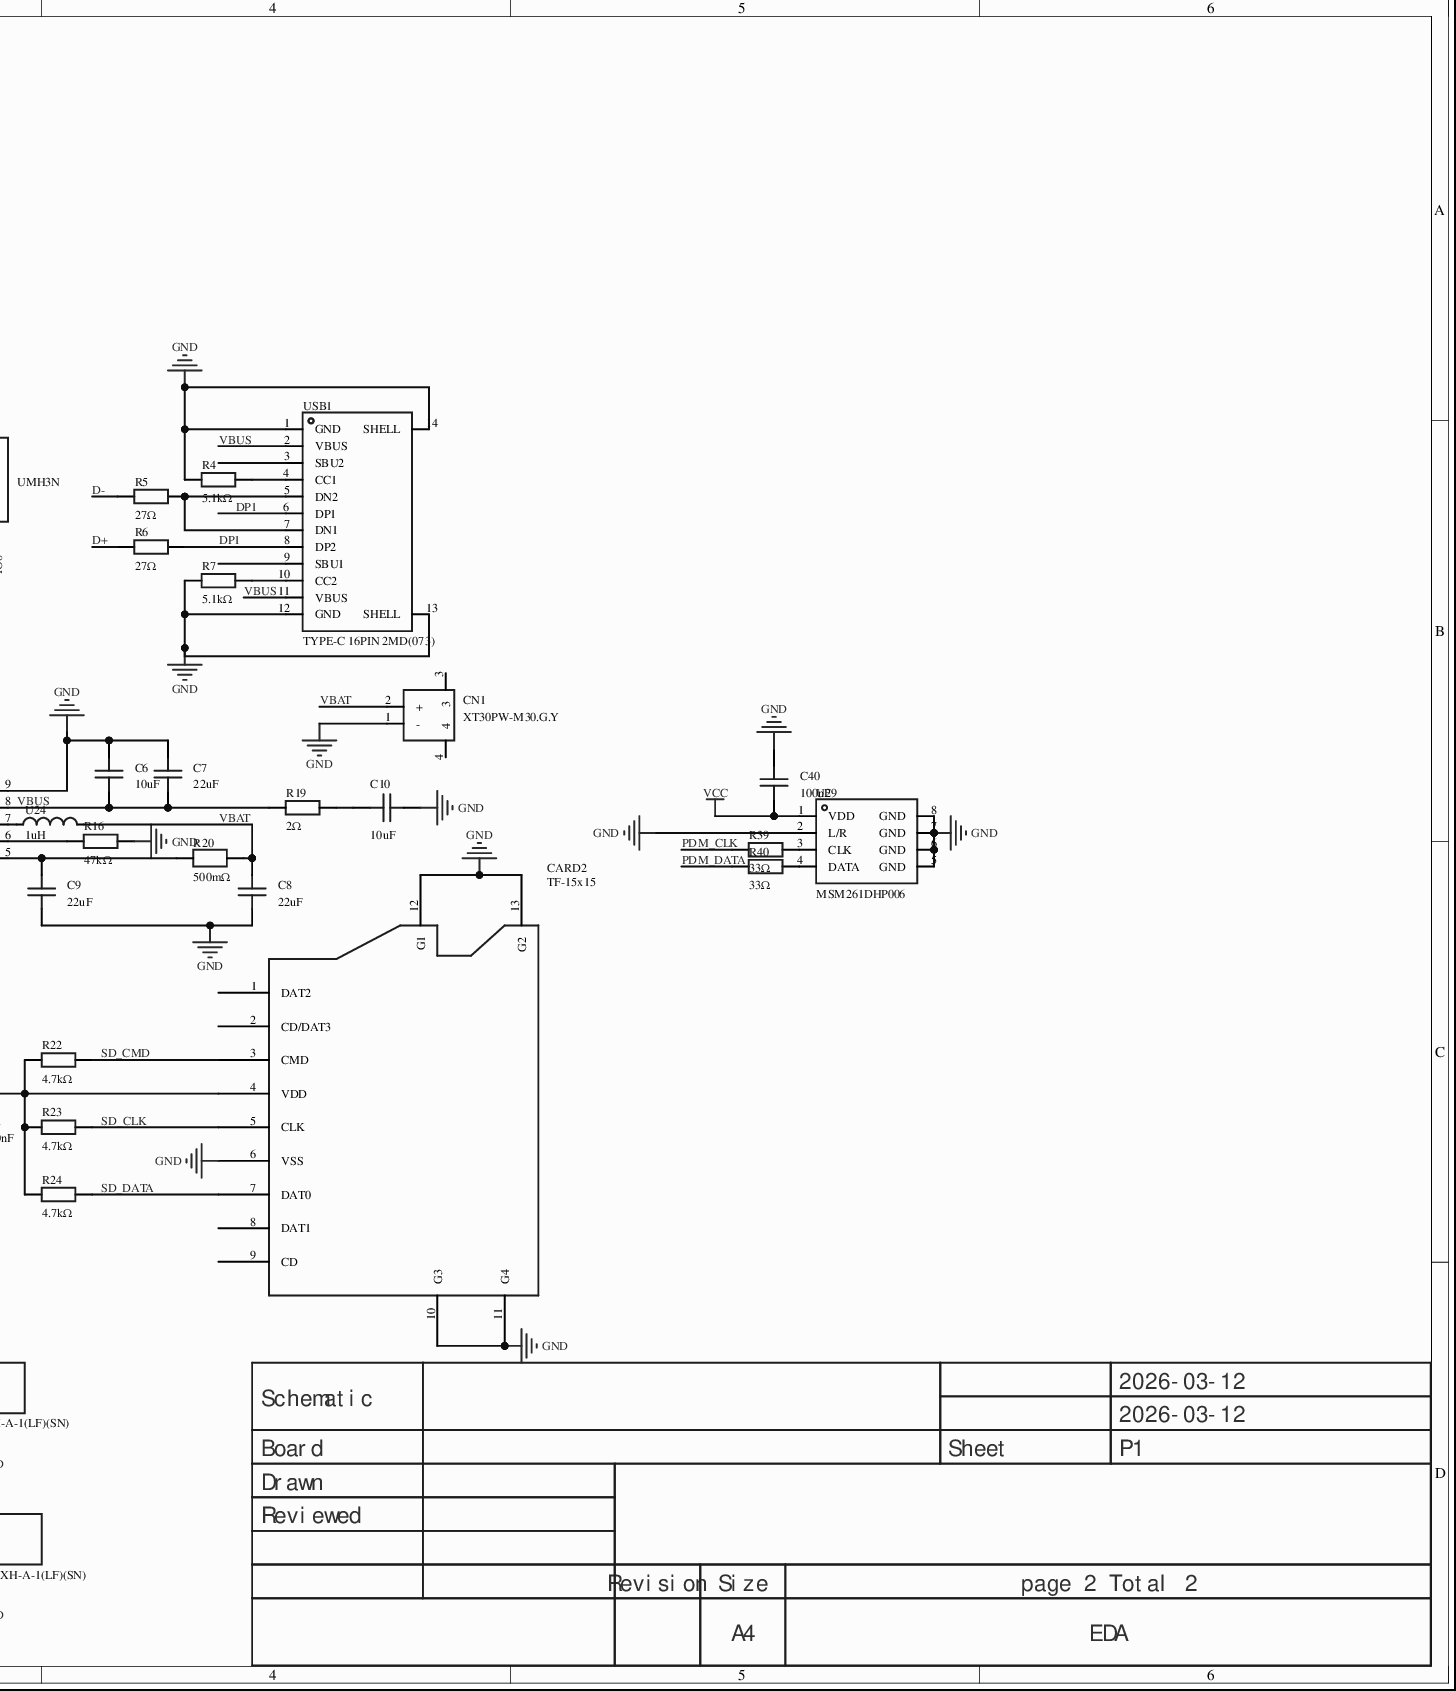
[diagram p0: MISC75432-3.schdoc, right]
# Altium project MISC75432-2.PrjPcb (part 2 of 3)

## Sheet MISC75432-3.schdoc (continued)

### Library data of the parts
C4 C5 = CL10C220JB8NNNC: Capacitance: 22pF; Tolerance: ±5%; Rated voltage: 50V; Temp. coefficient: C0G;; Manufacturer: SAMSUNG(三星); Add into BOM: yes; 3D Model: ac125912035d415993ca9572d50418b1; 3D Model Transform: 62.992,31.496,0,0,0,0,0,0,0; ModelName: C0603_L1.6-W0.8-H0.8; Symbol: CL10C220JB8NNNC; Device: CL10C220JB8NNNC; Convert to PCB: yes; Supplier Footprint: 0603; Value: 22pF; LCSC Part Name: 22pF ±5% 50V; Supplier Part: C1653; Manufacturer Part: CL10C220JB8NNNC; JLCPCB Part Class: Basic Part; Datasheet: https://example.com/datasheet/CL10C220JB8NNNC/2005.html; Supplier: LCSC; Voltage Rating: 50V; Temperature Coefficient: C0G; FootprintName: C0603
C6 C10 C15 C31 = CL10A106MA8NRNC: Capacitance: 10uF; Tolerance: ±20%; Rated voltage: 25V; Temp. coefficient: X5R;; Manufacturer: SAMSUNG(三星); Add into BOM: yes; 3D Model: ac125912035d415993ca9572d50418b1; 3D Model Transform: 62.992,31.496,0,0,0,0,0,0,0; ModelName: C0603_L1.6-W0.8-H0.8; Symbol: CL10A106MA8NRNC; Device: CL10A106MA8NRNC; Convert to PCB: yes; Supplier Footprint: 0603; Value: 10uF; LCSC Part Name: 10uF ±20% 25V; Supplier Part: C96446; Manufacturer Part: CL10A106MA8NRNC; JLCPCB Part Class: Basic Part; Datasheet: https://example.com/datasheet/CL10A106MA8NRNC/97651.html; Supplier: LCSC; Voltage Rating: 25V; Temperature Coefficient: X5R; FootprintName: C0603
C7-C9 C20 = CGA0603X5R226M160JT: Capacitance: 22uF; Tolerance: ±20%; Rated voltage: 16V; Temp. coefficient: X5R;; Manufacturer: HRE(芯声); Add into BOM: yes; 3D Model: ac125912035d415993ca9572d50418b1; 3D Model Transform: 62.992,31.496,0,0,0,0,0,0,0; ModelName: C0603_L1.6-W0.8-H0.8; Symbol: CGA0603X5R226M160JT; Device: CGA0603X5R226M160JT; Convert to PCB: yes; Supplier Footprint: 0603; Value: 22uF; LCSC Part Name: 22uF ±20% 16V; Supplier Part: C6119868; Manufacturer Part: CGA0603X5R226M160JT; JLCPCB Part Class: Extended Part; Datasheet: https://example.com/datasheet/CGA0603X5R226M160JT/7062574.html; Supplier: LCSC; Voltage Rating: 16V; Temperature Coefficient: X5R; FootprintName: C0603
C11 C12 C16 C18 C26 C32 C40 = CGA0603X7R104K500JT: Capacitance: 100nF; Tolerance: ±10%; Rated voltage: 50V; Temp. coefficient: X7R;; Manufacturer: HRE(芯声); Add into BOM: yes; 3D Model: ac125912035d415993ca9572d50418b1; 3D Model Transform: 62.992,31.496,0,0,0,0,0,0,0; ModelName: C0603_L1.6-W0.8-H0.8; Symbol: CGA0603X7R104K500JT; Device: CGA0603X7R104K500JT; Convert to PCB: yes; Supplier Footprint: 0603; Value: 100nF; LCSC Part Name: 100nF ±10% 50V; Supplier Part: C6119867; Manufacturer Part: CGA0603X7R104K500JT; JLCPCB Part Class: Extended Part; Datasheet: https://example.com/datasheet/CGA0603X7R104K500JT/7062573.html; Supplier: LCSC; Voltage Rating: 50V; Temperature Coefficient: X7R; FootprintName: C0603
C13 C14 C19 C27 C28 = CL10A105KB8NNNC: Capacitance: 1uF; Tolerance: ±10%; Rated voltage: 50V; Temp. coefficient: X5R;; Manufacturer: SAMSUNG(三星); Add into BOM: yes; 3D Model: ac125912035d415993ca9572d50418b1; 3D Model Transform: 62.992,31.496,0,0,0,0,0,0,0; ModelName: C0603_L1.6-W0.8-H0.8; Symbol: CL10A105KB8NNNC; Device: CL10A105KB8NNNC; Convert to PCB: yes; Supplier Footprint: 0603; Value: 1uF; LCSC Part Name: 1uF ±10% 50V; Supplier Part: C15849; Manufacturer Part: CL10A105KB8NNNC; JLCPCB Part Class: Basic Part; Datasheet: https://example.com/datasheet/CL10A105KB8NNNC/16531.html; Supplier: LCSC; Voltage Rating: 50V; Temperature Coefficient: X5R; FootprintName: C0603
C17 = RYHV50V2.2UF5*5: Capacitance: 2.2uF; Tolerance: ±20%; Rated voltage: 50V; Type: Polymer;; Manufacturer: HONOR(荣誉); Add into BOM: yes; 3D Model: ed942b427de741e3aabba01c64b2d723; 3D Model Transform: 236.22,208.661,0,0,0,0,-0.001,-0.003,0; Lifetime: 2000hrs@105℃; Symbol: RYHV50V2.2UF5*5; Device: RYHV50V2.2UF5*5; Convert to PCB: yes; Supplier Footprint: SMD,D5xL5.8mm; Value: 2.2uF; LCSC Part Name: 2.2uF ±20% 50V; Supplier Part: C48970657; Manufacturer Part: RYHV50V2.2UF5*5; JLCPCB Part Class: Extended Part; Datasheet: https://example.com/datasheet/RYHV50V2.2UF5*5/51295601.html; Supplier: LCSC; Voltage Rating: 50V; Type: Polymer; Diameter: 5mm; Height - Seated (Max): 5.8mm; Operating Temperature: -55℃~+105℃; FootprintName: CAP-SMD_BD5.0-L5.3-W5.3-LS6.0-FD; ModelName: CAP-SMD_BD5.0-L5.3-W5.3-LS6.0-FD
C21 = CL10C330JB8NNNC: Capacitance: 33pF; Tolerance: ±5%; Rated voltage: 50V; Temp. coefficient: C0G;; Manufacturer: SAMSUNG(三星); Add into BOM: yes; 3D Model: ac125912035d415993ca9572d50418b1; 3D Model Transform: 62.992,31.496,0,0,0,0,0,0,0; ModelName: C0603_L1.6-W0.8-H0.8; Symbol: CL10C330JB8NNNC; Device: CL10C330JB8NNNC; Convert to PCB: yes; Supplier Footprint: 0603; Value: 33pF; LCSC Part Name: 33pF ±5% 50V; Supplier Part: C1663; Manufacturer Part: CL10C330JB8NNNC; JLCPCB Part Class: Basic Part; Datasheet: https://example.com/datasheet/CL10C330JB8NNNC/2015.html; Supplier: LCSC; Voltage Rating: 50V; Temperature Coefficient: C0G; FootprintName: C0603
C22 = CL10B473KB8NNNC: Capacitance: 47nF; Tolerance: ±10%; Rated voltage: 50V; Temp. coefficient: X7R;; Manufacturer: SAMSUNG(三星); Add into BOM: yes; 3D Model: ac125912035d415993ca9572d50418b1; 3D Model Transform: 62.992,31.496,0,0,0,0,0,0,0; ModelName: C0603_L1.6-W0.8-H0.8; Symbol: CL10B473KB8NNNC; Device: CL10B473KB8NNNC; Convert to PCB: yes; Supplier Footprint: 0603; Value: 47nF; LCSC Part Name: 47nF ±10% 50V; Supplier Part: C1622; Manufacturer Part: CL10B473KB8NNNC; JLCPCB Part Class: Basic Part; Datasheet: https://example.com/datasheet/CL10B473KB8NNNC/1974.html; Supplier: LCSC; Voltage Rating: 50V; Temperature Coefficient: X7R; FootprintName: C0603
C23-C25 = RVT25V22M5X5: Capacitance: 22uF; Tolerance: ±20%; Rated voltage: 25V; Ripple current: 26mA@120Hz;; Manufacturer: JIERR(捷而瑞); AddInBom: yes; ModelId: 95a10e3217cd46fe9ce33b4e001305500819f05c4eef4c71ace90d822a990e87; ModelTransform: 224.409,208.661,0,0,0,0,0,0,0; Lifetime: 2000hrs@105℃; Symbol: RVT25V22M5X5; Device: RVT25V22M5X5; LCSC Part Name: 22uF ±20% 25V; SupplierPart: C47023110; ManufacturerPart: RVT25V22M5X5; Supplier Footprint: SMD,D5xL5.4mm; JLCPCB Part Class: Extended Part; Datasheet: https://example.com/datasheet/RVT25V22M5X5/49206211.html; Supplier: LCSC; ConvertToPcb: yes; FootprintName: CAP-SMD_BD5.0-L5.3-W5.3-LS6.3-FD-1; ModelName: CAP-SMD_BD5.0-L5.3-W5.3-LS6.3-FD-1; Value: 22uF; Voltage Rating: 25V; Ripple Current: 26mA@120Hz; Diameter: 5mm; Height - Seated (Max): 5.4mm; Operating Temperature: -55℃~+105℃
C29 = JVJ25V220M6x8: Capacitance: 220uF; Tolerance: ±20%; Rated voltage: 25V; Ripple current: 120mA@120Hz;; Manufacturer: JIERR(捷而瑞); AddInBom: yes; ModelId: ccbda52dceed4b139172c40f75c9da3f0819f05c4eef4c71ace90d822a990e87; ModelTransform: 287.401,259.842,0,0,0,0,0,0,0; Lifetime: 2000hrs@105℃; Symbol: JVJ25V220M6X8; Device: JVJ25V220M6x8; LCSC Part Name: 220uF ±20% 25V; SupplierPart: C46550404; ManufacturerPart: JVJ25V220M6x8; Supplier Footprint: SMD,D6.3xL7.7mm; JLCPCB Part Class: Extended Part; Datasheet: https://example.com/datasheet/JVJ25V220M6x8/48680098.html; Supplier: LCSC; ConvertToPcb: yes; FootprintName: CAP-SMD_BD6.3-L6.6-W6.6-LS7.3-FD-H7.7; ModelName: CAP-SMD_BD6.3-L6.6-W6.6-LS7.3-FD-H7.7; Value: 220uF; Voltage Rating: 25V; Ripple Current: 120mA@120Hz; Diameter: 6.3mm; Height - Seated (Max): 7.7mm; Operating Temperature: -55℃~+105℃
C30 C37-C39 = CC0603KRX7R7BB684: Capacitance: 680nF; Tolerance: ±10%; Rated voltage: 16V; Temp. coefficient: X7R;; Manufacturer: YAGEO(国巨); Add into BOM: yes; 3D Model: ac125912035d415993ca9572d50418b1; 3D Model Transform: 62.992,31.496,0,0,0,0,0,0,0; ModelName: C0603_L1.6-W0.8-H0.8; Symbol: CC0603KRX7R7BB684; Device: CC0603KRX7R7BB684; Convert to PCB: yes; Supplier Footprint: 0603; Value: 680nF; LCSC Part Name: 680nF ±10% 16V; Supplier Part: C107067; Manufacturer Part: CC0603KRX7R7BB684; JLCPCB Part Class: Extended Part; Datasheet: https://example.com/datasheet/CC0603KRX7R7BB684/108283.html; Supplier: LCSC; Voltage Rating: 16V; Temperature Coefficient: X7R; FootprintName: C0603
C33-C36 = CL10B224KA8NNNC: Capacitance: 220nF; Tolerance: ±10%; Rated voltage: 25V; Temp. coefficient: X7R;; Manufacturer: SAMSUNG(三星); Add into BOM: yes; 3D Model: ac125912035d415993ca9572d50418b1; 3D Model Transform: 62.992,31.496,0,0,0,0,0,0,0; ModelName: C0603_L1.6-W0.8-H0.8; Symbol: CL10B224KA8NNNC; Device: CL10B224KA8NNNC; Convert to PCB: yes; Supplier Footprint: 0603; Value: 220nF; LCSC Part Name: 220nF ±10% 25V; Supplier Part: C21120; Manufacturer Part: CL10B224KA8NNNC; JLCPCB Part Class: Basic Part; Datasheet: https://example.com/datasheet/CL10B224KA8NNNC/21832.html; Supplier: LCSC; Voltage Rating: 25V; Temperature Coefficient: X7R; FootprintName: C0603
C41 = CL10B102KB8NNNC: Capacitance: 1nF; Tolerance: ±10%; Rated voltage: 50V; Temp. coefficient: X7R;; Manufacturer: SAMSUNG(三星); Add into BOM: yes; 3D Model: ac125912035d415993ca9572d50418b1; 3D Model Transform: 62.992,31.496,0,0,0,0,0,0,0; ModelName: C0603_L1.6-W0.8-H0.8; Symbol: CL10B102KB8NNNC; Device: CL10B102KB8NNNC; Convert to PCB: yes; Supplier Footprint: 0603; Value: 1nF; LCSC Part Name: 1nF ±10% 50V; Supplier Part: C1588; Manufacturer Part: CL10B102KB8NNNC; JLCPCB Part Class: Basic Part; Datasheet: https://example.com/datasheet/CL10B102KB8NNNC/1940.html; Supplier: LCSC; Voltage Rating: 50V; Temperature Coefficient: X7R; FootprintName: C0603
CARD2 = TF-15x15: Card connection: Self-ejecting; Card type: MicroSD card (TF card); Connector type: Socket; Max body height: 2mm; Operating temp.: -25℃~+85℃;; Manufacturer: SOFNG(硕方); Symbol: TF-15×15; AddInBom: yes; ModelId: 67496f576e2f431c95a797a452f0eadc0819f05c4eef4c71ace90d822a990e87; ModelTransform: 598.424,635.826,0,0,0,0,79.804,8.934,-23.622; Device: TF-15x15; LCSC Part Name: 自弹式 MicroSD卡(TF卡) 卡座; SupplierPart: C111196; ManufacturerPart: TF-15x15; Supplier Footprint: SMD; JLCPCB Part Class: Extended Part; Datasheet: https://example.com/datasheet/TF-15x15/112422.html; Supplier: LCSC; ConvertToPcb: yes; FootprintName: TF-SMD_TF-15-15; ModelName: TF-SMD_TF-15-15; Card Connection Mode: Self-ejecting; Card Type: MicroSD card (TF card); Connector Type: Socket; Additional Card Detection Pins: Yes; Height Above Board: 2mm; Operating Temperature: -25℃~+85℃
CN1 = XT30PW-M30.G.Y: Socket,DCsupply,XT30,male,PIN:2; Manufacturer: AMASS(艾迈斯); AddInBom: yes; ModelId: 722652c2597f41cd937322584dc4b29b0819f05c4eef4c71ace90d822a990e87; ModelTransform: 523.621,549.2115,0,0,0,0,-0.005,-39.568,-78.74; Rated current: 15A; Rated voltage: 500VDC; Connector type: RC model plug; Wire gauge: 16/18/20AWG; contact resistance: 1.2mΩ; Symbol: XT30PW-M; Device: XT30PW-M30.G.Y; LCSC Part Name: AMASS(艾迈斯)航模插头 卧式弯脚 XT30PW-M公头; SupplierPart: C431092; ManufacturerPart: XT30PW-M30.G.Y; Supplier Footprint: -; JLCPCB Part Class: Extended Part; Datasheet: https://example.com/datasheet/XT30PW-M30.G.Y/426930.html; Supplier: LCSC; ConvertToPcb: yes; FootprintName: CONN-TH_XT30PW-M; ModelName: CONN-TH_XT30PW-M; Size/Specification: 2pin; interface form: Male
CN2 CN3 = S2B-XH-A-1(LF)(SN): Pin structure: 1x2P; Pitch: 2.5mm; Mounting: Right-angle THT; Series: XH; Total pins: 2P; Rows: 1; Pins per row: 2; Row spacing: -; Rated current: 3A; Contact material: Brass; Contact plating: Tin; Operating temp.: -25℃~+85℃;; Manufacturer: JST; AddInBom: yes; ModelId: 91927f2a0f7340abaa498c02c76d9b390819f05c4eef4c71ace90d822a990e87; ModelTransform: 291.338,452.755,0,0,0,0,0.394,73.43,-129.921; Number of PINs Per Row: 2; Voltage Rating: 250V; Plastic Material: PA66; Flame Retardant Rating: UL94V-0; Supplementary Features: Kinked pins; Z-Height of the Board: 6.1mm; X-Length of Bottom Edge on Board (Spacing Line): 7.4mm; Y-Width of Bottom Edge on Board: 11.5mm; Symbol: S2B-XH-A-1 (LF)(SN); Device: S2B-XH-A-1(LF)(SN); LCSC Part Name: 1x2P 间距:2.5mm 弯插 系列:XH; SupplierPart: C163035; ManufacturerPart: S2B-XH-A-1(LF)(SN); Supplier Footprint: 弯插,P=2.5mm; JLCPCB Part Class: Extended Part; Datasheet: https://example.com/datasheet/S2B-XH-A-1(LF)(SN)/174416.html; Supplier: LCSC; ConvertToPcb: yes; FootprintName: CONN-TH_S2B-XH-A-1-LF-SN; ModelName: CONN-TH_S2B-XH-A-1-LF-SN; Pins Structure: 1x2P; Mounting Type: Right-angle THT; Reference Series: XH; Number of Pins: 2P; Number of Rows: 1; Row Spacing: -; Current Rating: 3A; Contact Material: Brass; Contact Plating: Tin; Operating Temperature: -25℃~+85℃; Color: White
D1 D2 = 1N4148W_C7420318: Diode configuration: Discrete; Forward voltage drop (Vf): 1.25V@150mA; DC reverse voltage (Vr): 100V; Rectified current: 150mA; Reverse recovery time (Trr): 4ns;; Manufacturer: R+O(宏嘉诚); AddInBom: yes; ModelId: 5054d9b7be8b429dad093a54b517b4dd0819f05c4eef4c71ace90d822a990e87; ModelTransform: 145.669,61.024,0,0,0,0,0,0,0; Pd - Power Dissipation: 400mW; Reverse Leakage Current (Ir): 1uA@75V; Operating Junction Temperature Range: -55℃~+150℃; Non-Repetitive Peak Forward Surge Current: 2A; Symbol: 1N4148W_C7420318; Device: 1N4148W_C7420318; LCSC Part Name: 100V 150mA; SupplierPart: C7420318; ManufacturerPart: 1N4148W; Supplier Footprint: SOD-123; JLCPCB Part Class: Extended Part; Datasheet: https://example.com/datasheet/1N4148W/8397140.html; Supplier: LCSC; ConvertToPcb: yes; FootprintName: SOD-123_L2.7-W1.6-LS3.7-FD; ModelName: SOD-123_L2.7-W1.6-LS3.7-FD; Diode Configuration: Discrete; Voltage - Forward(Vf@If): 1.25V@150mA; Voltage - DC Reverse(Vr): 100V; Current - Rectified: 150mA; Reverse Recovery Time (trr): 4ns
L1 = SRG0420-2R2-M: Inductance: 2.2uH; Tolerance: ±20%; Rated current: 4A; Saturation current (Isat): 5A; Type: Molded inductor;; Manufacturer: JIERR(捷而瑞); AddInBom: yes; DC Resistance(DCR): 49mΩ; Symbol: SRG0420-2R2-M; Device: SRG0420-2R2-M; LCSC Part Name: 2.2μH ±20% 5A; SupplierPart: C53462916; ManufacturerPart: SRG0420-2R2-M; Supplier Footprint: SMD,4.6x4.1mm; JLCPCB Part Class: Extended Part; Datasheet: https://example.com/datasheet/SRG0420-2R2-M/56628161.html; Supplier: LCSC; ConvertToPcb: yes; FootprintName: IND-SMD_L4.6-W4.1_MHCI04015; Value: 2.2uH; Current Rating: 4A; Current - Saturation(Isat): 5A; Type: Molded inductor
L2-L5 = FXL0630-100-M: Inductance: 10uH; Tolerance: ±20%; Rated current: 4.5A; Saturation current (Isat): 5.5A; Type: Molded inductor;; Manufacturer: cjiang(长江微电); AddInBom: yes; ModelId: e28854526ca747668ea12fbe1dd39a630819f05c4eef4c71ace90d822a990e87; ModelName: IND-SMD_L7.3-W6.8-H3.0; ModelTransform: 292.125,267.716,0,0,0,0,0,0,0; DC Resistance(DCR): 68mΩ; Symbol: FXL0630-100-M; Device: FXL0630-100-M; LCSC Part Name: 10uH ±20% 5.5A; SupplierPart: C167223; ManufacturerPart: FXL0630-100-M; Supplier Footprint: SMD,7x6.6mm; JLCPCB Part Class: Extended Part; Datasheet: https://example.com/datasheet/FXL0630-100-M/178606.html; Supplier: LCSC; ConvertToPcb: yes; FootprintName: IND-SMD_L7.3-W6.8; Value: 10uH; Current Rating: 4.5A; Current - Saturation(Isat): 5.5A; Type: Molded inductor; Ratings: -
LED1 LED2 = NCD0603Y2: Emitted color: Yellow; Forward voltage (VF): 1.6V~2.6V; Power: 65mW; Forward current: 20mA; Dominant wavelength: 586nm~595nm; Lens color: Clear lens; Luminous intensity: 100mcd~220mcd; Viewing angle: 130°; Operating temp.: -30℃~+85℃;; Manufacturer: 国星光电; Symbol: FC-1608YXK-585F08; AddInBom: yes; ModelId: 1f0d29a91be547639d425604e9b96ebb0819f05c4eef4c71ace90d822a990e87; ModelTransform: 63.7794,32.283,0,0,0,0,0,0,0; Device: NCD0603Y2; LCSC Part Name: NCD0603Y2; SupplierPart: C89811; ManufacturerPart: NCD0603Y2; Supplier Footprint: 0603; JLCPCB Part Class: Extended Part; Datasheet: https://example.com/upload/public/pdf/source/20200820/C89811_7FE84B429B6BCA3E113B125EE1452576.pdf; Supplier: LCSC; ConvertToPcb: yes; FootprintName: LED0603-RD; ModelName: LED0603-RD; Emitted Color: Yellow; Forward Voltage (VF): 1.6V~2.6V; Power Dissipation: 65mW; Forward Current: 20mA; Dominant Wavelength: 586nm~595nm; Lens Color: Clear lens; Luminous Intensity: 100mcd~220mcd; Viewing Angle: 130°; Operating Temperature: -30℃~+85℃
Q17 = UMH3N: Quantity: -; Collector-emitter breakdown voltage (Vceo): 50V; Collector current (Ic): 100mA; Power dissipation (Pd): 150mW; DC current gain (hFE): 100@1mA,5V;; Manufacturer: CJ(江苏长电/长晶); AddInBom: yes; ModelId: 7779600a2eb94c6fae04993c10cd58cb0819f05c4eef4c71ace90d822a990e87; ModelName: SC-70-6_L2.0-W1.3-H1.0-P0.65; ModelTransform: 82.677,78.74,0,0,0,0,0,0,0; Input Resistor: 6.11kΩ; Symbol: UMH3N; Device: UMH3N; LCSC Part Name: 数字晶体管（内置电阻）; SupplierPart: C62892; ManufacturerPart: UMH3N; Supplier Footprint: SOT-363; JLCPCB Part Class: Extended Part; Datasheet: https://example.com/datasheet/UMH3N/63955.html; Supplier: LCSC; ConvertToPcb: yes; FootprintName: SC-70-6_L2.2-W1.3-P0.65-LS2.1-BR; Number: -; Collector - Emitter Voltage VCEO: 50V; Current - Collector(Ic): 100mA; Pd - Power Dissipation: 150mW; DC Current Gain: 100@1mA,5V; Emitter-Base Voltage VEBO: 5V; Operating Temperature: -55℃~+150℃
Q18 = 2N7002_C8545: Quantity: 1 N-channel; Drain-source voltage (Vdss): 60V; Continuous drain current (Id): 115mA; On-resistance (RDS(on)): 5Ω@10V; Power dissipation (Pd): 225mW; Threshold voltage (Vgs(th)): 2.5V;; Manufacturer: CJ(江苏长电/长晶); 3D Model: c62791f0466c4ae2a892c056b845b0ca0819f05c4eef4c71ace90d822a990e87; 3D Model Transform: 98.425,114.173,0,180,0,0,0.0005,-0.0005,0; Input Capacitance(Ciss): 50pF; Reverse Transfer Capacitance (Crss@Vds): 5pF; AddInBom: yes; ModelName: SOT-23-3P_L2.9-W1.3-H1.0-LS2.4-P0.95; Symbol: 2N7002; Device: 2N7002_C8545; LCSC Part Name: 1个N沟道 耐压:60V 电流:115mA; Supplier Part: C8545; Manufacturer Part: 2N7002; Supplier Footprint: SOT-23; JLCPCB Part Class: Basic Part; Datasheet: https://example.com/datasheet/2N7002/9040.html; Supplier: LCSC; Number: 1 N-channel; Drain to Source Voltage: 60V; Current - Continuous Drain(Id): 115mA; RDS(on): 5Ω@10V; Pd - Power Dissipation: 225mW; Gate Threshold Voltage (Vgs(th)): 2.5V; Operating Temperature: -; ConvertToPcb: yes; FootprintName: SOT-23-3_L2.9-W1.3-P1.90-LS2.4-BR
R3 R13 R26 R34 R36 = 0603WAF1002T5E: Resistor type: Thick-film; Resistance: 10kΩ; Tolerance: ±1%; Power: 100mW; Working voltage: 75V; Temp. coefficient: ±100ppm/℃;; Manufacturer: UNI-ROYAL(厚声); Add into BOM: yes; 3D Model: fc143cca1e79419f9cd78b61e9279f08; 3D Model Transform: 31.8897,63.7794,0,90,0,0,0,0,0; Symbol: 0603WAF1002T5E; Device: 0603WAF1002T5E; Convert to PCB: yes; Supplier Footprint: 0603; Value: 10kΩ; LCSC Part Name: 厚膜电阻 10kΩ ±1% 100mW; Supplier Part: C25804; Manufacturer Part: 0603WAF1002T5E; JLCPCB Part Class: Basic Part; Datasheet: https://example.com/datasheet/0603WAF1002T5E/26547.html; Supplier: LCSC; Type: Thick-film resistor; Power(Watts): 100mW; Voltage-Supply(Max): 75V; Temperature Coefficient: ±100ppm/℃; Operating Temperature: -55℃~+155℃; FootprintName: R0603; ModelName: R0603
R4 R7 = 0603WAF5101T5E: Resistor type: Thick-film; Resistance: 5.1kΩ; Tolerance: ±1%; Power: 100mW; Working voltage: 75V; Temp. coefficient: ±100ppm/℃;; Manufacturer: UNI-ROYAL(厚声); Add into BOM: yes; 3D Model: fc143cca1e79419f9cd78b61e9279f08; 3D Model Transform: 31.8897,63.7794,0,90,0,0,0,0,0; Symbol: 0603WAF5101T5E; Device: 0603WAF5101T5E; Convert to PCB: yes; Supplier Footprint: 0603; Value: 5.1kΩ; LCSC Part Name: 5.1kΩ ±1% 100mW 厚膜电阻; Supplier Part: C23186; Manufacturer Part: 0603WAF5101T5E; JLCPCB Part Class: Basic Part; Datasheet: https://example.com/datasheet/0603WAF5101T5E/23913.html; Supplier: LCSC; Type: Thick-film resistor; Power(Watts): 100mW; Voltage-Supply(Max): 75V; Temperature Coefficient: ±100ppm/℃; Operating Temperature: -55℃~+155℃; FootprintName: R0603; ModelName: R0603
R5 R6 = 0603WAF270JT5E: Resistor type: Thick-film; Resistance: 27Ω; Tolerance: ±1%; Power: 100mW; Working voltage: 75V; Temp. coefficient: ±200ppm/℃;; Manufacturer: UNI-ROYAL(厚声); Add into BOM: yes; 3D Model: fc143cca1e79419f9cd78b61e9279f08; 3D Model Transform: 31.8897,63.7794,0,90,0,0,0,0,0; Symbol: 0603WAF270JT5E; Device: 0603WAF270JT5E; Convert to PCB: yes; Supplier Footprint: 0603; Value: 27Ω; LCSC Part Name: 27Ω ±1% 100mW 厚膜电阻; Supplier Part: C25190; Manufacturer Part: 0603WAF270JT5E; JLCPCB Part Class: Extended Part; Datasheet: https://example.com/datasheet/0603WAF270JT5E/25933.html; Supplier: LCSC; Type: Thick-film resistor; Power(Watts): 100mW; Voltage-Supply(Max): 75V; Temperature Coefficient: ±200ppm/℃; Operating Temperature: -55℃~+155℃; FootprintName: R0603; ModelName: R0603
R8-R12 = FRC0603F49R9TS: Resistor type: Thick-film; Resistance: 49.9Ω; Tolerance: ±1%; Power: 100mW; Working voltage: 75V; Temp. coefficient: ±100ppm/℃;; Manufacturer: FOJAN(富捷); Add into BOM: yes; 3D Model: fc143cca1e79419f9cd78b61e9279f08; 3D Model Transform: 31.8897,63.7794,0,90,0,0,0,0,0; Symbol: FRC0603F49R9TS; Device: FRC0603F49R9TS; Convert to PCB: yes; Supplier Footprint: 0603; Value: 49.9Ω; LCSC Part Name: 49.9Ω ±1% 100mW 厚膜电阻; Supplier Part: C2930110; Manufacturer Part: FRC0603F49R9TS; JLCPCB Part Class: Extended Part; Supplier: LCSC; Type: Thick-film resistor; Power(Watts): 100mW; Voltage-Supply(Max): 75V; Temperature Coefficient: ±100ppm/℃; Operating Temperature: -55℃~+155℃; FootprintName: R0603; ModelName: R0603
R14 = 0603WAF1001T5E: Resistor type: Thick-film; Resistance: 1kΩ; Tolerance: ±1%; Power: 100mW; Working voltage: 75V; Temp. coefficient: ±100ppm/℃;; Manufacturer: UNI-ROYAL(厚声); Add into BOM: yes; 3D Model: fc143cca1e79419f9cd78b61e9279f08; 3D Model Transform: 31.8897,63.7794,0,90,0,0,0,0,0; Symbol: 0603WAF1001T5E; Device: 0603WAF1001T5E; Convert to PCB: yes; Supplier Footprint: 0603; Value: 1kΩ; LCSC Part Name: 1kΩ ±1% 100mW 厚膜电阻; Supplier Part: C21190; Manufacturer Part: 0603WAF1001T5E; JLCPCB Part Class: Basic Part; Datasheet: https://example.com/datasheet/0603WAF1001T5E/21904.html; Supplier: LCSC; Type: Thick-film resistor; Power(Watts): 100mW; Voltage-Supply(Max): 75V; Temperature Coefficient: ±100ppm/℃; Operating Temperature: -55℃~+155℃; FootprintName: R0603; ModelName: R0603
R15 = 0603WAF8202T5E: Resistor type: Thick-film; Resistance: 82kΩ; Tolerance: ±1%; Power: 100mW; Working voltage: 75V; Temp. coefficient: ±100ppm/℃;; Manufacturer: UNI-ROYAL(厚声); Add into BOM: yes; 3D Model: fc143cca1e79419f9cd78b61e9279f08; 3D Model Transform: 31.8897,63.7794,0,90,0,0,0,0,0; Symbol: 0603WAF8202T5E; Device: 0603WAF8202T5E; Convert to PCB: yes; Supplier Footprint: 0603; Value: 82kΩ; LCSC Part Name: 82kΩ ±1% 100mW 厚膜电阻; Supplier Part: C23254; Manufacturer Part: 0603WAF8202T5E; JLCPCB Part Class: Basic Part; Datasheet: https://example.com/datasheet/0603WAF8202T5E/23981.html; Supplier: LCSC; Type: Thick-film resistor; Power(Watts): 100mW; Voltage-Supply(Max): 75V; Temperature Coefficient: ±100ppm/℃; Operating Temperature: -55℃~+155℃; FootprintName: R0603; ModelName: R0603
R16 = 0603WAF4702T5E: Resistor type: Thick-film; Resistance: 47kΩ; Tolerance: ±1%; Power: 100mW; Working voltage: 75V; Temp. coefficient: ±100ppm/℃;; Manufacturer: UNI-ROYAL(厚声); Add into BOM: yes; 3D Model: fc143cca1e79419f9cd78b61e9279f08; 3D Model Transform: 31.8897,63.7794,0,90,0,0,0,0,0; Symbol: 0603WAF4702T5E; Device: 0603WAF4702T5E; Convert to PCB: yes; Supplier Footprint: 0603; Value: 47kΩ; LCSC Part Name: 47kΩ ±1% 100mW 厚膜电阻; Supplier Part: C25819; Manufacturer Part: 0603WAF4702T5E; JLCPCB Part Class: Basic Part; Datasheet: https://example.com/datasheet/0603WAF4702T5E/26562.html; Supplier: LCSC; Type: Thick-film resistor; Power(Watts): 100mW; Voltage-Supply(Max): 75V; Temperature Coefficient: ±100ppm/℃; Operating Temperature: -55℃~+155℃; FootprintName: R0603; ModelName: R0603
R17 R21 = 0603WAF1000T5E: Resistor type: Thick-film; Resistance: 100Ω; Tolerance: ±1%; Power: 100mW; Max working voltage: 75V; Temp. coefficient: ±200ppm/℃;; Manufacturer: UNI-ROYAL(厚声); Add into BOM: yes; 3D Model: fc143cca1e79419f9cd78b61e9279f08; 3D Model Transform: 31.8897,63.7794,0,90,0,0,0,0,0; Symbol: 0603WAF1000T5E; Device: 0603WAF1000T5E; Convert to PCB: yes; Supplier Footprint: 0603; Value: 100Ω; LCSC Part Name: 100Ω ±1% 100mW 厚膜电阻; Supplier Part: C22775; Manufacturer Part: 0603WAF1000T5E; JLCPCB Part Class: Basic Part; Datasheet: https://example.com/upload/public/pdf/source/20200306/C422600_1E6D84923E4A46A82E41ADD87F860B5C.pdf; Supplier: LCSC; Type: Thick-film resistor; Power(Watts): 100mW; Overload Voltage (Max): 75V; Temperature Coefficient: ±200ppm/℃; Operating Temperature Range: -55℃~+155℃; FootprintName: R0603; ModelName: R0603
R18 = HNTC0805-104F3950FB: Resistance: 100kΩ; B value (25℃/50℃): 3950K; Resistance tolerance: ±1%; Power: 200mW; B value tolerance: ±1%; Max steady-state current (25℃): 140uA;; Manufacturer: R+O(宏嘉诚); AddInBom: yes; ModelId: 37a81e68749a4138bd2dfa6897b24b850819f05c4eef4c71ace90d822a990e87; ModelName: R0805_L2.0-W1.3-H0.6; ModelTransform: 78.74,51.181,0,0,0,0,0,-0.0005,0; Dissipation Factor: 2mW/℃; Thermal Time Constant: 5s; Pitch: 0.5mm; Symbol: HNTC0805-104F3950FB; Device: HNTC0805-104F3950FB; LCSC Part Name: HNTC0805-104F3950FB; SupplierPart: C49247664; ManufacturerPart: HNTC0805-104F3950FB; Supplier Footprint: 0805; JLCPCB Part Class: Extended Part; Datasheet: https://example.com/datasheet/HNTC0805-104F3950FB/51678317.html; Supplier: LCSC; ConvertToPcb: yes; FootprintName: R0805; Resistance @ 25℃: 100kΩ; B Constant (25℃/50℃): 3950K; Resistance Tolerance: ±1%; Power(Watts): 200mW; B Constant Tolerance: ±1%; Steady State Current (Max): 140uA; Operating Temperature: -40℃~+125℃; Length: 2mm; Width: 1.25mm; Height: 0.85mm
R19 = RC0603FR-072RL: Resistor type: Thick-film; Resistance: 2Ω; Tolerance: ±1%; Power: 100mW; Max working voltage: 75V; Temp. coefficient: ±200ppm/℃;; Manufacturer: YAGEO(国巨); Add into BOM: yes; 3D Model: fc143cca1e79419f9cd78b61e9279f08; 3D Model Transform: 31.8897,63.7794,0,90,0,0,0,0,0; Symbol: RC0603FR-072RL; Device: RC0603FR-072RL; Convert to PCB: yes; Supplier Footprint: 0603; Value: 2Ω; LCSC Part Name: 厚膜电阻 2Ω ±1% 100mW; Supplier Part: C185341; Manufacturer Part: RC0603FR-072RL; JLCPCB Part Class: Extended Part; Datasheet: https://example.com/upload/public/pdf/source/20180904/C276339_014E484F1DBA106FB92D45EABD5A1AC1.pdf; Supplier: LCSC; Type: Thick-film resistor; Power(Watts): 100mW; Overload Voltage (Max): 75V; Temperature Coefficient: ±200ppm/℃; Operating Temperature Range: -55℃~+155℃; FootprintName: R0603; ModelName: R0603
R20 = HoJLRH1206-1W-500mR-1%: Resistor type: Thin-film; Resistance: 500mΩ; Tolerance: ±1%; Power: 1W; Temp. coefficient: ±100ppm/℃;; Manufacturer: Milliohm(毫欧); AddInBom: yes; ModelId: 89a1f13db2384da588040e0b3c55bf660819f05c4eef4c71ace90d822a990e87; ModelName: R1206_L3.2-W1.6-H0.6; ModelTransform: 125.984,62.992,0,0,0,0,0,0,0; Symbol: HOJLRH1206-1W-500MR-1%; Device: HoJLRH1206-1W-500mR-1%; LCSC Part Name: 薄膜电阻 500mΩ ±1% 1W; SupplierPart: C46594303; ManufacturerPart: HoJLRH1206-1W-500mR-1%; Supplier Footprint: 1206; Datasheet: https://example.com/datasheet/HoJLRH1206-1W-500mR-1%2525/48731416.html; Supplier: LCSC; ConvertToPcb: yes; FootprintName: R1206; Type: Thin-film resistor; Value: 500mΩ; Power(Watts): 1W; Temperature Coefficient: ±100ppm/℃; Operating Temperature: -55℃~+155℃
R22-R24 R35 = 0603WAF4701T5E: Resistor type: Thick-film; Resistance: 4.7kΩ; Tolerance: ±1%; Power: 100mW; Working voltage: 75V; Temp. coefficient: ±100ppm/℃;; Manufacturer: UNI-ROYAL(厚声); Add into BOM: yes; 3D Model: fc143cca1e79419f9cd78b61e9279f08; 3D Model Transform: 31.8897,63.7794,0,90,0,0,0,0,0; Symbol: 0603WAF4701T5E; Device: 0603WAF4701T5E; Convert to PCB: yes; Supplier Footprint: 0603; Value: 4.7kΩ; LCSC Part Name: 4.7kΩ ±1% 100mW 厚膜电阻; Supplier Part: C23162; Manufacturer Part: 0603WAF4701T5E; JLCPCB Part Class: Basic Part; Datasheet: https://example.com/datasheet/0603WAF4701T5E/23889.html; Supplier: LCSC; Type: Thick-film resistor; Power(Watts): 100mW; Voltage-Supply(Max): 75V; Temperature Coefficient: ±100ppm/℃; Operating Temperature: -55℃~+155℃; FootprintName: R0603; ModelName: R0603
R25 = 0603WAF1004T5E: Resistor type: Thick-film; Resistance: 1MΩ; Tolerance: ±1%; Power: 100mW; Max working voltage: 75V; Temp. coefficient: ±100ppm/℃;; Manufacturer: UNI-ROYAL(厚声); Add into BOM: yes; 3D Model: fc143cca1e79419f9cd78b61e9279f08; 3D Model Transform: 31.8897,63.7794,0,90,0,0,0,0,0; Symbol: 0603WAF1004T5E; Device: 0603WAF1004T5E; Convert to PCB: yes; Supplier Footprint: 0603; Value: 1MΩ; LCSC Part Name: 1MΩ ±1% 100mW 厚膜电阻; Supplier Part: C22935; Manufacturer Part: 0603WAF1004T5E; JLCPCB Part Class: Basic Part; Datasheet: https://example.com/upload/public/pdf/source/20200306/C422600_1E6D84923E4A46A82E41ADD87F860B5C.pdf; Supplier: LCSC; Type: Thick-film resistor; Power(Watts): 100mW; Overload Voltage (Max): 75V; Temperature Coefficient: ±100ppm/℃; Operating Temperature Range: -55℃~+155℃; FootprintName: R0603; ModelName: R0603
R27 R29 R33 = 0603WAF1003T5E: Resistor type: Thick-film; Resistance: 100kΩ; Tolerance: ±1%; Power: 100mW; Working voltage: 75V; Temp. coefficient: ±100ppm/℃;; Manufacturer: UNI-ROYAL(厚声); Add into BOM: yes; 3D Model: fc143cca1e79419f9cd78b61e9279f08; 3D Model Transform: 31.8897,63.7794,0,90,0,0,0,0,0; Symbol: 0603WAF1003T5E; Device: 0603WAF1003T5E; Convert to PCB: yes; Supplier Footprint: 0603; Value: 100kΩ; LCSC Part Name: 100kΩ ±1% 100mW 厚膜电阻; Supplier Part: C25803; Manufacturer Part: 0603WAF1003T5E; JLCPCB Part Class: Basic Part; Datasheet: https://example.com/datasheet/0603WAF1003T5E/26546.html; Supplier: LCSC; Type: Thick-film resistor; Power(Watts): 100mW; Voltage-Supply(Max): 75V; Temperature Coefficient: ±100ppm/℃; Operating Temperature: -55℃~+155℃; FootprintName: R0603; ModelName: R0603
R28 = 0603WAF4993T5E: Resistor type: Thick-film; Resistance: 499kΩ; Tolerance: ±1%; Power: 100mW; Working voltage: 75V; Temp. coefficient: ±100ppm/℃;; Manufacturer: UNI-ROYAL(厚声); Add into BOM: yes; 3D Model: fc143cca1e79419f9cd78b61e9279f08; 3D Model Transform: 31.8897,63.7794,0,90,0,0,0,0,0; Symbol: 0603WAF4993T5E; Device: 0603WAF4993T5E; Convert to PCB: yes; Supplier Footprint: 0603; Value: 499kΩ; LCSC Part Name: 499kΩ ±1% 100mW 厚膜电阻; Supplier Part: C26751; Manufacturer Part: 0603WAF4993T5E; JLCPCB Part Class: Extended Part; Datasheet: https://example.com/datasheet/0603WAF4993T5E/27497.html; Supplier: LCSC; Type: Thick-film resistor; Power(Watts): 100mW; Voltage-Supply(Max): 75V; Temperature Coefficient: ±100ppm/℃; Operating Temperature: -55℃~+155℃; FootprintName: R0603; ModelName: R0603
R30 = 0603WAF2493T5E: Resistor type: Thick-film; Resistance: 249kΩ; Tolerance: ±1%; Power: 100mW; Working voltage: 75V; Temp. coefficient: ±100ppm/℃;; Manufacturer: UNI-ROYAL(厚声); Add into BOM: yes; 3D Model: fc143cca1e79419f9cd78b61e9279f08; 3D Model Transform: 31.8897,63.7794,0,90,0,0,0,0,0; Symbol: 0603WAF2493T5E; Device: 0603WAF2493T5E; Convert to PCB: yes; Supplier Footprint: 0603; Value: 249kΩ; LCSC Part Name: 249kΩ ±1% 100mW 厚膜电阻; Supplier Part: C22918; Manufacturer Part: 0603WAF2493T5E; JLCPCB Part Class: Extended Part; Datasheet: https://example.com/datasheet/0603WAF2493T5E/23645.html; Supplier: LCSC; Type: Thick-film resistor; Power(Watts): 100mW; Voltage-Supply(Max): 75V; Temperature Coefficient: ±100ppm/℃; Operating Temperature: -55℃~+155℃; FootprintName: R0603; ModelName: R0603
R31 = 0603WAF2002T5E: Resistor type: Thick-film; Resistance: 20kΩ; Tolerance: ±1%; Power: 100mW; Working voltage: 75V; Temp. coefficient: ±100ppm/℃;; Manufacturer: UNI-ROYAL(厚声); Add into BOM: yes; 3D Model: fc143cca1e79419f9cd78b61e9279f08; 3D Model Transform: 31.8897,63.7794,0,90,0,0,0,0,0; Symbol: 0603WAF2002T5E; Device: 0603WAF2002T5E; Convert to PCB: yes; Supplier Footprint: 0603; Value: 20kΩ; LCSC Part Name: 20kΩ ±1% 100mW 厚膜电阻; Supplier Part: C4184; Manufacturer Part: 0603WAF2002T5E; JLCPCB Part Class: Basic Part; Datasheet: https://example.com/datasheet/0603WAF2002T5E/4591.html; Supplier: LCSC; Type: Thick-film resistor; Power(Watts): 100mW; Voltage-Supply(Max): 75V; Temperature Coefficient: ±100ppm/℃; Operating Temperature: -55℃~+155℃; FootprintName: R0603; ModelName: R0603
R32 = 0603WAF1803T5E: Resistor type: Thick-film; Resistance: 180kΩ; Tolerance: ±1%; Power: 100mW; Working voltage: 75V; Temp. coefficient: ±100ppm/℃;; Manufacturer: UNI-ROYAL(厚声); Add into BOM: yes; 3D Model: fc143cca1e79419f9cd78b61e9279f08; 3D Model Transform: 31.8897,63.7794,0,90,0,0,0,0,0; Symbol: 0603WAF1803T5E; Device: 0603WAF1803T5E; Convert to PCB: yes; Supplier Footprint: 0603; Value: 180kΩ; LCSC Part Name: 180kΩ ±1% 100mW 厚膜电阻; Supplier Part: C22827; Manufacturer Part: 0603WAF1803T5E; JLCPCB Part Class: Extended Part; Datasheet: https://example.com/datasheet/0603WAF1803T5E/23554.html; Supplier: LCSC; Type: Thick-film resistor; Power(Watts): 100mW; Voltage-Supply(Max): 75V; Temperature Coefficient: ±100ppm/℃; Operating Temperature: -55℃~+155℃; FootprintName: R0603; ModelName: R0603
R37 R38 = 0603WAF2201T5E: Resistor type: Thick-film; Resistance: 2.2kΩ; Tolerance: ±1%; Power: 100mW; Max working voltage: 75V; Temp. coefficient: ±100ppm/℃;; Manufacturer: UNI-ROYAL(厚声); Add into BOM: yes; 3D Model: fc143cca1e79419f9cd78b61e9279f08; 3D Model Transform: 31.8897,63.7794,0,90,0,0,0,0,0; Symbol: 0603WAF2201T5E; Device: 0603WAF2201T5E; Convert to PCB: yes; Supplier Footprint: 0603; Value: 2.2kΩ; LCSC Part Name: 2.2kΩ ±1% 100mW 厚膜电阻; Supplier Part: C4190; Manufacturer Part: 0603WAF2201T5E; JLCPCB Part Class: Basic Part; Datasheet: https://example.com/upload/public/pdf/source/20200306/C422600_1E6D84923E4A46A82E41ADD87F860B5C.pdf; Supplier: LCSC; Type: Thick-film resistor; Power(Watts): 100mW; Overload Voltage (Max): 75V; Temperature Coefficient: ±100ppm/℃; Operating Temperature Range: -55℃~+155℃; FootprintName: R0603; ModelName: R0603
R39 R40 = 0603WAF330JT5E: Resistor type: Thick-film; Resistance: 33Ω; Tolerance: ±1%; Power: 100mW; Working voltage: 75V; Temp. coefficient: ±100ppm/℃;; Manufacturer: UNI-ROYAL(厚声); Add into BOM: yes; 3D Model: fc143cca1e79419f9cd78b61e9279f08; 3D Model Transform: 31.8897,63.7794,0,90,0,0,0,0,0; Symbol: 0603WAF330JT5E; Device: 0603WAF330JT5E; Convert to PCB: yes; Supplier Footprint: 0603; Value: 33Ω; LCSC Part Name: 33Ω ±1% 100mW 厚膜电阻; Supplier Part: C23140; Manufacturer Part: 0603WAF330JT5E; JLCPCB Part Class: Basic Part; Datasheet: https://example.com/datasheet/0603WAF330JT5E/23867.html; Supplier: LCSC; Type: Thick-film resistor; Power(Watts): 100mW; Voltage-Supply(Max): 75V; Temperature Coefficient: ±100ppm/℃; Operating Temperature: -55℃~+155℃; FootprintName: R0603; ModelName: R0603
SW1 SW2 = TS-1088-AR02016: Circuit: SPST; Button shape: Round; Actuating force: 1.6N; Mounting: Upright SMD; Switch length: 4mm; Switch width: 3mm; Switch height: 2mm; Bracket: Without bracket; Contact current: 50mA; Rated voltage: 12V; Life: 10万 cycles;; Manufacturer: XUNPU(讯普); AddInBom: yes; ModelId: b26698b69f274ffabef8a26c7d0e5dd10819f05c4eef4c71ace90d822a990e87; ModelName: SW-SMD_L3.9-W2.9-H2.0-LS4.8; ModelTransform: 188.976,114.174,0,0,0,0,0,0,0; Actuator Style: Round button; Actuator/Cap Color: Black; Symbol: TS-1088-AR02016; Device: TS-1088-AR02016; LCSC Part Name: 4*3*2mm 立贴 轻触开关; SupplierPart: C720477; ManufacturerPart: TS-1088-AR02016; Supplier Footprint: SMD,4x3mm; JLCPCB Part Class: Basic Part; Datasheet: https://example.com/datasheet/TS-1088-AR02016/763484.html; Supplier: LCSC; ConvertToPcb: yes; FootprintName: SW-SMD_L3.9-W3.0-P4.45; Operating Force: 1.6N; Mounting Type: Upright SMD; Length: 4mm; Width: 3mm; Switch Height: 2mm; with Bracket: Without bracket; Contact Current: 50mA; Voltage Rating: 12V; Termination Style: SMD tab; Life: 10万 cycles; Operating Temperature: -30℃~+80℃
SW3 = TS-1009B-05026: Circuit: SPST; Button shape: Round; Mounting: Right-angle THT; Switch length: 4.5mm; Switch width: 4.5mm; Switch height: 5mm; Contact current: 50mA; Rated voltage: 12V; LED: -; Life: -;; Manufacturer: XUNPU(讯普); Add into BOM: yes; 3D Model: 8eca28fb04ca48cca17ebf6c8f349844; 3D Model Transform: 177.165,196.85,0,0,0,0,0,-25.591,-78.74; Actuator Style: Round button; Symbol: TS-1009B-05026; Device: TS-1009B-05026; Convert to PCB: yes; LCSC Part Name: 4.5*4.5*5mm 卧插 轻触开关; Supplier Part: C455252; Manufacturer Part: TS-1009B-05026; Supplier Footprint: 插件,4.5x4.5mm; JLCPCB Part Class: Extended Part; Datasheet: https://example.com/datasheet/TS-1009B-05026/457607.html; Supplier: LCSC; Mounting Type: Right-angle THT; Length: 4.5mm; Width: 4.5mm; Switch Height: 5mm; Contact Current: 50mA; Voltage Rating: 12V; Life: -; With Lamp: -; FootprintName: SW-TH_3P-L4.5-W3.8-P3.10-LS1.9_TS-1009B-05026; ModelName: SW-TH_3P-L4.5-W3.8-P3.10-LS1.9_TS-1009B-05026
U2 = CH340G: Application: USB to UART; Interface protocol: USB 2.0; Data rate: 2Mbps;; Manufacturer: WCH(南京沁恒); AddInBom: yes; ModelId: c21ec766ec2643efb3352f8441994f4e0819f05c4eef4c71ace90d822a990e87; ModelName: SOIC-16_L9.9-W3.9-H1.8-LS6.0-P1.27; ModelTransform: 389.763,236.454,0,0,0,0,0,0,0; Protocol: USB 2.0; Supply Voltage: 5V; 3.3V; Symbol: CH340G; Device: CH340G; LCSC Part Name: USB转串口芯片CH340; SupplierPart: C14267; ManufacturerPart: CH340G; Supplier Footprint: SOP-16; JLCPCB Part Class: Extended Part; Datasheet: https://example.com/upload/public/pdf/source/20240313/8510303D24D987FBF1AD30058571F10E.pdf; Supplier: LCSC; ConvertToPcb: yes; FootprintName: SOIC-16_L9.9-W3.9-P1.27-LS6.0-BL; Applications Function: USB to UART; Data Rate: 2Mbps; Operating Temperature: -40℃~+85℃
U15 = ESP32-S3-WROOM-1-N8R8: Manufacturer: ESPRESSIF(乐鑫); Symbol: ESP32-S3-WROOM-1(N8R8); 3D Model: 481f5bdfc076422c9bb3c23c3ada9c170819f05c4eef4c71ace90d822a990e87; 3D Model Transform: 708.73866,1003.97437,0,0,0,0,0,143.7,0; AddInBom: yes; Device: ESP32-S3-WROOM-1-N8R8; LCSC Part Name: ESP32-S3-WROOM-1-N8R8; Supplier Part: C2913201; Manufacturer Part: ESP32-S3-WROOM-1-N8R8; Supplier Footprint: SMD,25.5x18mm; JLCPCB Part Class: Extended Part; Datasheet: https://example.com/datasheet/ESP32-S3-WROOM-1-N8R8/3198299.html; Supplier: LCSC; ConvertToPcb: yes; FootprintName: WIRELM-SMD_ESP32-S3-WROOM-1; ModelName: WIRELM-SMD_ESP32-S3-WROOM-1
U23 = IP2312U_VSET: Working voltage: 4.5V~5.5V; Max charge current: 3A; Battery type: -; Battery cells: 1;; Manufacturer: INJOINIC(英集芯); Symbol: IP2312; AddInBom: yes; ModelId: 94c97984fe8342edbe821bc2ce85d11e0819f05c4eef4c71ace90d822a990e87; ModelName: SOP-8_L4.9-W3.9-H1.7-LS6.0-P1.30; ModelTransform: 236.22,839.658,0,90,0,0,0.0005,-0.0005,0; The Chip Type: Charger IC; Charging Saturation Voltage: 4.2V; Number of Cells: 1; Battery Temperature Detection: Supported; Supply Current (Iq): 50uA; Device: IP2312U_VSET; LCSC Part Name: 可调充满电压，通过1号脚调整 单节锂电池同步开关降压充电IC; SupplierPart: C605432; ManufacturerPart: IP2312U_VSET; Supplier Footprint: SOP-8-EP; JLCPCB Part Class: Extended Part; Datasheet: https://example.com/datasheet/IP2312U_VSET/635666.html; Supplier: LCSC; ConvertToPcb: yes; FootprintName: SOP-8_L4.9-W3.9-P1.27-LS6.0-BL-EP; Voltage - Supply: 4.5V~5.5V; Charge Current - Max: 3A; End-Off Voltage: -; Type of Battery: -; Operating Temperature: -40℃~+150℃
U24 = FTC252012S1R0MBCA: Inductance: 1uH; Tolerance: ±20%; Rated current: 4A; Saturation current (Isat): 5.6A; Type: -;; Manufacturer: cjiang(长江微电); AddInBom: yes; ModelId: e143e04106934774881cec608355723f0819f05c4eef4c71ace90d822a990e87; ModelTransform: 98.504,78.819,0,0,0,0,-0.004,-0.003,0; DC Resistance(DCR): 35mΩ; Symbol: FTC252012S1R0MBCA; Device: FTC252012S1R0MBCA; LCSC Part Name: 1uH ±20% 5.6A; SupplierPart: C5832370; ManufacturerPart: FTC252012S1R0MBCA; Supplier Footprint: 1008; JLCPCB Part Class: Extended Part; Datasheet: https://example.com/datasheet/FTC252012S1R0MBCA/6763490.html; Supplier: LCSC; ConvertToPcb: yes; FootprintName: IND-SMD_L2.5-W2.0-VLS252012CX-150M; ModelName: IND-SMD_L2.5-W2.0-VLS252012CX-150M; Value: 1uH; Current Rating: 4A; Current - Saturation(Isat): 5.6A; Type: -
U26 = ME6211A33M3G-N: Output type: Fixed; Working voltage: 6V; Output voltage: 3.3V; Output current: 500mA; PSRR: 70dB@(1kHz); Output polarity: Positive;; Manufacturer: MICRONE(南京微盟); AddInBom: yes; ModelId: 89cb27a44ab2466697082bb9fd73a7d00819f05c4eef4c71ace90d822a990e87; ModelName: SOT-23-3L_L2.9-W1.6-H1.1-LS2.8-P0.95; ModelTransform: 114.173,110.236,0,90,0,0,0,0,0; Voltage Dropout: 120mV@(100mA); standby current: 60uA; Noise: 50uVrms; Number of Outputs: 1; Symbol: ME6211A33M3G-N; Device: ME6211A33M3G-N; LCSC Part Name: 输入6V 输出3.3V 500mA; SupplierPart: C168807; ManufacturerPart: ME6211A33M3G-N; Supplier Footprint: SOT-23-3; JLCPCB Part Class: Extended Part; Datasheet: https://example.com/datasheet/ME6211A33M3G-N/180190.html; Supplier: LCSC; ConvertToPcb: yes; FootprintName: SOT-23-3_L2.9-W1.6-P1.90-LS2.8-BR; Output Type: Fixed; Voltage - Supply: 6V; Output Voltage: 3.3V; Output Current: 500mA; Power Supply Rejection Ratio (PSRR): 70dB@(1kHz); Features: Overcurrent protection; enable; short-circuit protection; Operating Temperature: -40℃~+150℃; Output Configuration: Positive
U27 = TAS5805MPWPR: Amplifier type: Class-D; Speaker channels: Stereo; Output power: 23W×2@8Ω; Quiescent current (Iq): 16.5mA;; Manufacturer: TI(德州仪器); AddInBom: yes; ModelId: c33b2f64442f42ecb27b91aed85c9e5a0819f05c4eef4c71ace90d822a990e87; ModelTransform: 381.889,251.968,0,0,0,0,0,0,0; Class: Class-D amplifier; Voltage - Supply: 4.5V~26.4V; Total Harmonic Distortion + Noise (THD+N): 0.03%; Signal-to-Noise Ratio: 107dB; Power Supply Rejection Ratio (PSRR): 72dB; Symbol: TAS5805MPWPR; Device: TAS5805MPWPR; LCSC Part Name: 23W立体声D类音频功率放大器; SupplierPart: C478472; ManufacturerPart: TAS5805MPWPR; Supplier Footprint: HTSSOP-28-EP; JLCPCB Part Class: Extended Part; Supplier: LCSC; ConvertToPcb: yes; FootprintName: HTSSOP-28_L9.7-W4.4-P0.65-LS6.4-BL-EP; ModelName: HTSSOP-28_L9.7-W4.4-P0.65-LS6.4-BL-EP; Speaker Channels: Stereo; Output Power: 23W×2@8Ω; Quiescent Current: 16.5mA; Operating Temperature: -25℃~+85℃
U28 = TPS61088RHLR: Function type: Boost; Output type: Adjustable; Working voltage: 2.7V~12V; Output voltage: 4.5V~12.6V; Output current: 10A;; Manufacturer: TI(德州仪器); AddInBom: yes; ModelId: 5fea786b771f49529c9badc1d7bb6c830819f05c4eef4c71ace90d822a990e87; ModelName: VQFN-20_L4.5-W3.5-H1.0-P0.50; ModelTransform: 177.952,138.5824,0,0,0,0,0.078,0,0; Switching Frequency: 200kHz~2.2MHz; Number of Outputs: 1; Switch tube (built-in/external): Built-in; Symbol: TPS61088RHLR; Device: TPS61088RHLR; LCSC Part Name: 全集成同步升压转换器; SupplierPart: C87357; ManufacturerPart: TPS61088RHLR; Supplier Footprint: VQFN-20-EP(3.6x4.6); JLCPCB Part Class: Extended Part; Supplier: LCSC; ConvertToPcb: yes; FootprintName: VQFN-20_L4.6-W3.6-P0.50-BL; Function: Boost; Output Type: Adjustable; Input Voltage: 2.7V~12V; Output Voltage: 4.5V~12.6V; Output Current: 10A; Operating Temperature: -40℃~+85℃; Synchronous Rectification: Yes; Topology: Boost; Quiescent Current (Iq): -
U29 = MSM261DHP006: Manufacturer: MEMS(敏芯微); AddInBom: yes; ModelId: a4d37d2771f348a097f021a1fa69af310819f05c4eef4c71ace90d822a990e87; ModelTransform: 118.11,157.48,0,0,0,0,0,0,0; Symbol: MSM261DHP006; Device: MSM261DHP006; LCSC Part Name: MSM261DHP006; SupplierPart: C22390138; ManufacturerPart: MSM261DHP006; Supplier Footprint: LGA-8(3x4); JLCPCB Part Class: Extended Part; Datasheet: https://example.com/datasheet/MSM261DHP006/23962951.html; Supplier: LCSC; ConvertToPcb: yes; FootprintName: QFN-8_L4.0-W3.0_WMM7040DTHN0-8-TR; ModelName: QFN-8_L4.0-W3.0_WMM7040DTHN0-8-TR
U30 = TPS22965DSGR: Type: Load switch; Channels: 1; Input control logic: Active high; Max continuous current: 6A; Working voltage: 800mV~5.7V; On-resistance: 16mΩ;; Manufacturer: TI(德州仪器); AddInBom: yes; ModelId: 946e25d6e4b040a1926ac3aab630211e0819f05c4eef4c71ace90d822a990e87; ModelName: UDFN-8_L2.0-W2.0-H0.8-P0.50; ModelTransform: 78.74,77.96,0,0,0,0,0,0,0; Number of Channels: 1; Symbol: TPS22965DSGR; Device: TPS22965DSGR; LCSC Part Name: 5.7V，6A，超低导通电阻负载开关; SupplierPart: C122837; ManufacturerPart: TPS22965DSGR; Supplier Footprint: UDFN-8-EP(2x2); JLCPCB Part Class: Extended Part; Supplier: LCSC; ConvertToPcb: yes; FootprintName: UDFN-8_L2.0-W2.0-P0.50-TL-EP; Control Input Logic: Active high; Maximum Continuous Current: 6A; Voltage - Supply: 800mV~5.7V; RDS(on): 16mΩ; Operating Temperature	-: -40℃~+85℃
USB1 = TYPE-C 16PIN 2MD(073): Connector type: Type-C; Protocol standard: -; Gender: Female; Mounting: Horizontal SMD; Contacts: 16P; Ports: 1; Rated current - power: 3A; Operating temp.: -25℃~+85℃;; Manufacturer: SHOU HAN(首韩); AddInBom: yes; ModelId: 3a41b9ec9b654a0fad4d118405ec62900819f05c4eef4c71ace90d822a990e87; ModelTransform: 351.9678,298.4246,0,0,0,0,0,-47.244,-35.433; Number of Ports: 1; Voltage Rating: 5V; Connect-Disconnect Life: 5千 cycles; Detection color: Black; Symbol: TYPE-C 16PIN 2MD(073); Device: TYPE-C 16PIN 2MD(073); LCSC Part Name: 16P卧贴母座; SupplierPart: C2765186; ManufacturerPart: TYPE-C 16PIN 2MD(073); Supplier Footprint: SMD; JLCPCB Part Class: Extended Part; Datasheet: https://example.com/datasheet/TYPE-C%252016PIN%25202MD(073)/2901843.html; Supplier: LCSC; ConvertToPcb: yes; FootprintName: USB-C-SMD_TYPE-C-6PIN-2MD-073; ModelName: USB-C-SMD_TYPE-C-6PIN-2MD-073; Connector Type: Type-C; Protocol Standard: -; Mounting Type: Horizontal SMD; Number of Contacts: 16P; Current Rating-Power: 3A; Supplementary Features: -; Center Height: -; Length: -; Operating Temperature: -25℃~+85℃
X1 = X322512MSB4SI: Crystal type: SMD crystal; Frequency: 12MHz; Room-temp. frequency deviation: ±10ppm; Load capacitance: 20pF; Frequency stability: ±20ppm;; Manufacturer: YXC(扬兴晶振); AddInBom: yes; ModelId: ff2dfd5650294453a14147960efe18380819f05c4eef4c71ace90d822a990e87; ModelTransform: 125.984,98.425,0,0,0,0,0,0,0; Symbol: X322512MSB4SI; Device: X322512MSB4SI; LCSC Part Name: YSX321SL 12MHZ 4P 3225 20PF ±10PPM -40~85℃ (±20PPM); SupplierPart: C9002; ManufacturerPart: X322512MSB4SI; Supplier Footprint: SMD3225-4P; JLCPCB Part Class: Basic Part; Datasheet: https://example.com/datasheet/X322512MSB4SI/9522.html; Supplier: LCSC; ConvertToPcb: yes; FootprintName: CRYSTAL-SMD_4P-L3.2-W2.5-BL; ModelName: CRYSTAL-SMD_4P-L3.2-W2.5-BL; Type: SMD crystal; Value: 12MHz; Normal temperature Frequency Tolerance: ±10ppm; Load Capacitance: 20pF; Frequency Stability: ±20ppm; Operating Temperature: -40℃~+85℃